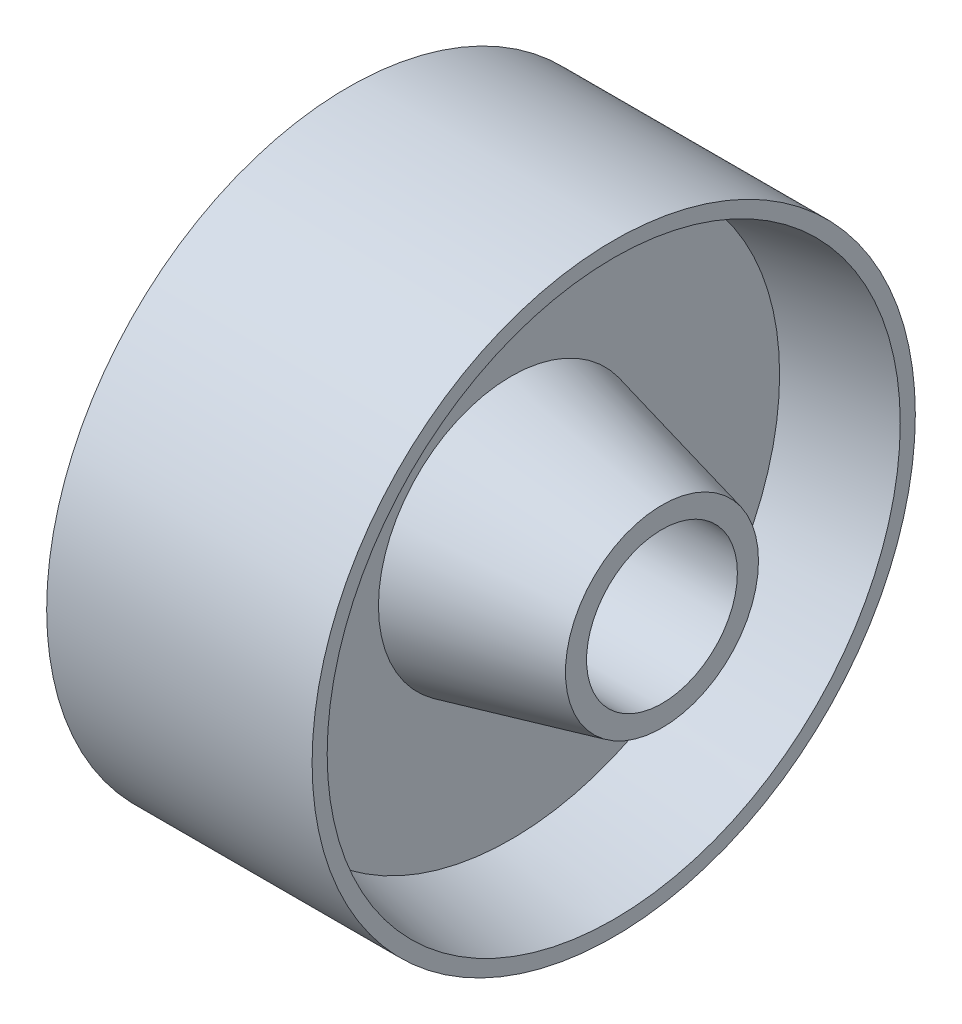
SolidWorks part; units mm, degrees
ref_plane "Front Plane" through (0, 0, 0) normal (0, 0, 1) x (1, 0, 0)
ref_plane "Top Plane" through (0, 0, 0) normal (0, 1, 0) x (1, 0, 0)
ref_plane "Right Plane" through (0, 0, 0) normal (1, 0, 0) x (0, 0, -1)
sketch "Sketch1" plane through (0, 0, 0) normal (0, 0, 1) x (1, 0, 0)
  line L0 (0, 0) -> (0, 2029.6657) construction
  line L1 (0, 0) -> (-2591.9815, 0) construction
  line L2 (-762, 317.5) -> (-762, 406.4)
  line L3 (-762, 406.4) -> (-127, 558.8)
  line L4 (-127, 558.8) -> (-127, 1130.3)
  line L5 (-127, 1130.3) -> (-558.8, 1206.5)
  line L6 (-558.8, 1206.5) -> (-558.8, 1270)
  line L7 (558.8, 1206.5) -> (558.8, 1270)
  line L8 (127, 1130.3) -> (558.8, 1206.5)
  line L9 (127, 558.8) -> (127, 1130.3)
  line L10 (762, 406.4) -> (127, 558.8)
  line L11 (762, 317.5) -> (762, 406.4)
  line L12 (-558.8, 1270) -> (558.8, 1270)
  line L13 (-762, 317.5) -> (762, 317.5)
  point P16 (0, 317.5)
  dimension "D1" = 317.5
  dimension "D2" = 88.9
  dimension "D3" = 152.4
  dimension "D4" = 571.5
  dimension "D5" = 76.2
  dimension "D6" = 63.5
  dimension "D7" = 1524
  dimension "D8" = 254
  dimension "D9" = 1117.6
revolve "Revolve1" add sketch "Sketch1" angle 360 about L1
